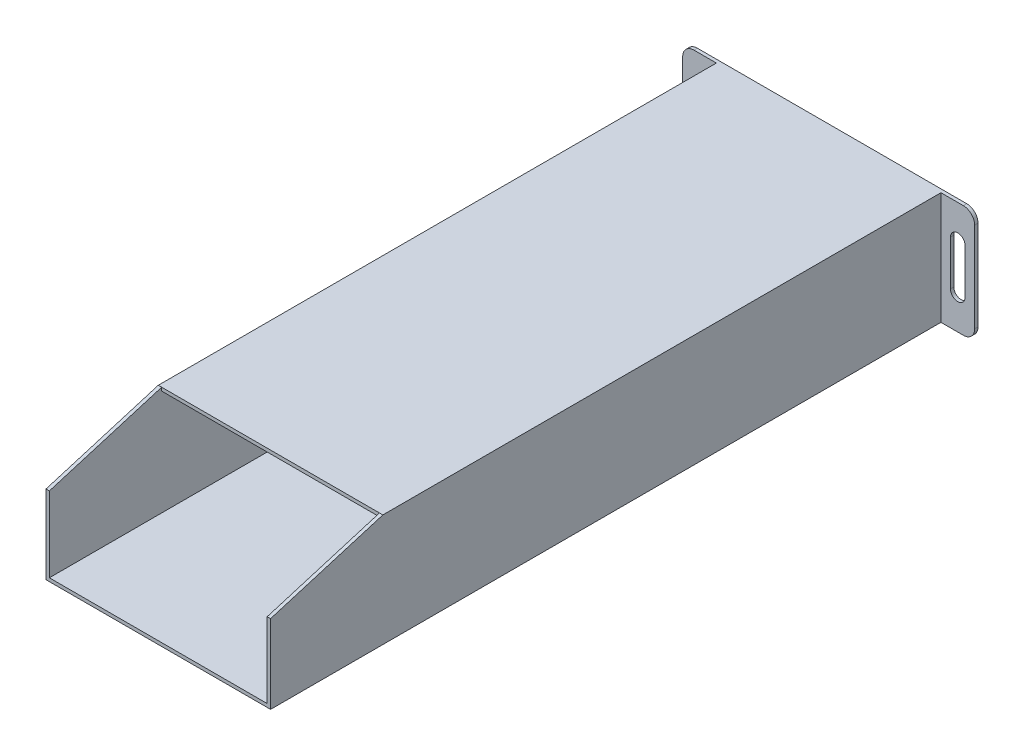
from build123d import *

# Parameters (mm, degrees)
SKETCH_14_W         = 100
SKETCH_14_H         = 50
EXTRUDE_1_DEPTH     = 300
SHELL_1_T           = -1.5
SKETCH_15_W         = 15
SKETCH_15_H         = 50
EXTRUDE_2_DEPTH     = 1.5
CUT_EXTRUDE_1_DEPTH = 323.257660886
FILLET_1_R          = 5
CUT_EXTRUDE_4_DEPTH = 307.51631278
CUT_EXTRUDE_5_REACH = 313.006
SKETCH_21_W         = 97
SKETCH_21_H         = 10


with BuildPart() as part:
    # 草图14 → 凸台-拉伸1 (new body)
    with BuildSketch(Plane.XY):
        Rectangle(SKETCH_14_W, SKETCH_14_H)
    extrude(amount=EXTRUDE_1_DEPTH)

    # 抽壳1
    shell_1_openings = [part.faces().sort_by_distance(p)[0] for p in [
        (0, 0, 300),
        (0, 0, 0),
    ]]
    offset(amount=SHELL_1_T, openings=shell_1_openings, kind=Kind.INTERSECTION)

    # 草图15 → 凸台-拉伸2 (add)
    with BuildSketch(Plane(origin=(0, 0, 0), x_dir=(-1, 0, 0), z_dir=(0, 0, -1))):
        with Locations((-57.5, 0)):
            Rectangle(SKETCH_15_W, SKETCH_15_H)
        with Locations((57.5, 0)):
            Rectangle(SKETCH_15_W, SKETCH_15_H)
    extrude(amount=-EXTRUDE_2_DEPTH)

    # 草图16 → 切除-拉伸1 (cut, through all)
    with BuildSketch(Plane(origin=(50, 0, 0), x_dir=(0, 0, -1), z_dir=(1, 0, 0))):
        Polygon((-300, 10), (-250, 25), (-300, 25), align=None)
    extrude(amount=-CUT_EXTRUDE_1_DEPTH, mode=Mode.SUBTRACT)

    # 圆角1
    fillet_1_edges = [part.edges().sort_by_distance(p)[0] for p in [
        (65, -25, 0.75),
        (65, 25, 0.75),
        (-65, 25, 0.75),
        (-65, -25, 0.75),
    ]]
    fillet(fillet_1_edges, radius=FILLET_1_R)

    # 草图20 → 切除-拉伸4 (cut, through all)
    with BuildSketch(Plane.XY.offset(1.5)):
        with BuildLine():
            Line((-60.75, -10), (-60.75, 10))
            ThreePointArc((-60.75, 10), (-57.5, 13.25), (-54.25, 10))
            Line((-54.25, 10), (-54.25, -10))
            ThreePointArc((-54.25, -10), (-57.5, -13.25), (-60.75, -10))
        make_face()
    cut_extrude_4 = extrude(amount=-CUT_EXTRUDE_4_DEPTH, mode=Mode.SUBTRACT)

    # 镜向1: 切除-拉伸4 across plane
    add(cut_extrude_4.mirror(Plane(origin=(0, 0, 0), x_dir=(0, 0, 1), z_dir=(1, 0, 0))), mode=Mode.SUBTRACT)

    # 草图21 → 切除-拉伸5 (cut, up to next)
    with BuildSketch(Plane(origin=(0, 25, 0), x_dir=(1, 0, 0), z_dir=(0, 1, 0)), mode=Mode.PRIVATE) as cut_extrude_5_sk1:
        with Locations((0, -255)):
            Rectangle(SKETCH_21_W, SKETCH_21_H)
    cut_extrude_5_tool1 = extrude(cut_extrude_5_sk1.sketch, amount=-CUT_EXTRUDE_5_REACH, mode=Mode.PRIVATE) & part.part
    add(cut_extrude_5_tool1.solids().sort_by_distance((0, 25, 255))[0], mode=Mode.SUBTRACT)


solid = part.part
